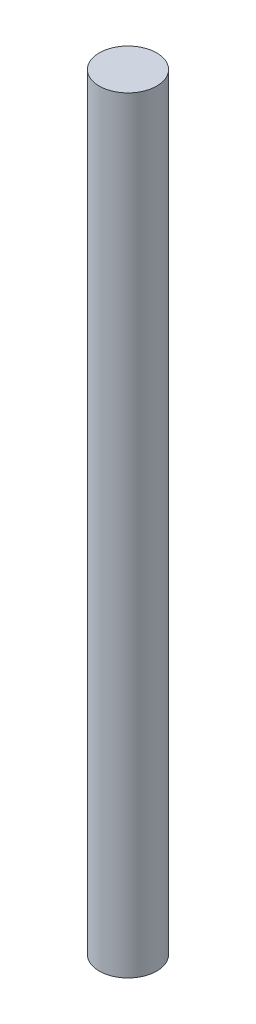
SolidWorks part; units mm, degrees
ref_plane "Front Plane" through (0, 0, 0) normal (0, 0, 1) x (1, 0, 0)
ref_plane "Top Plane" through (0, 0, 0) normal (0, 1, 0) x (1, 0, 0)
ref_plane "Right Plane" through (0, 0, 0) normal (1, 0, 0) x (0, 0, -1)
other "Configuration Table"
sketch "Sketch1" plane through (0, 0, 0) normal (0, 1, 0) x (1, 0, 0)
  circle A0 centre (0, 0) radius 90
  dimension "D1" = 180
extrude "Boss-Extrude1" add sketch "Sketch1" along normal blind 2400
